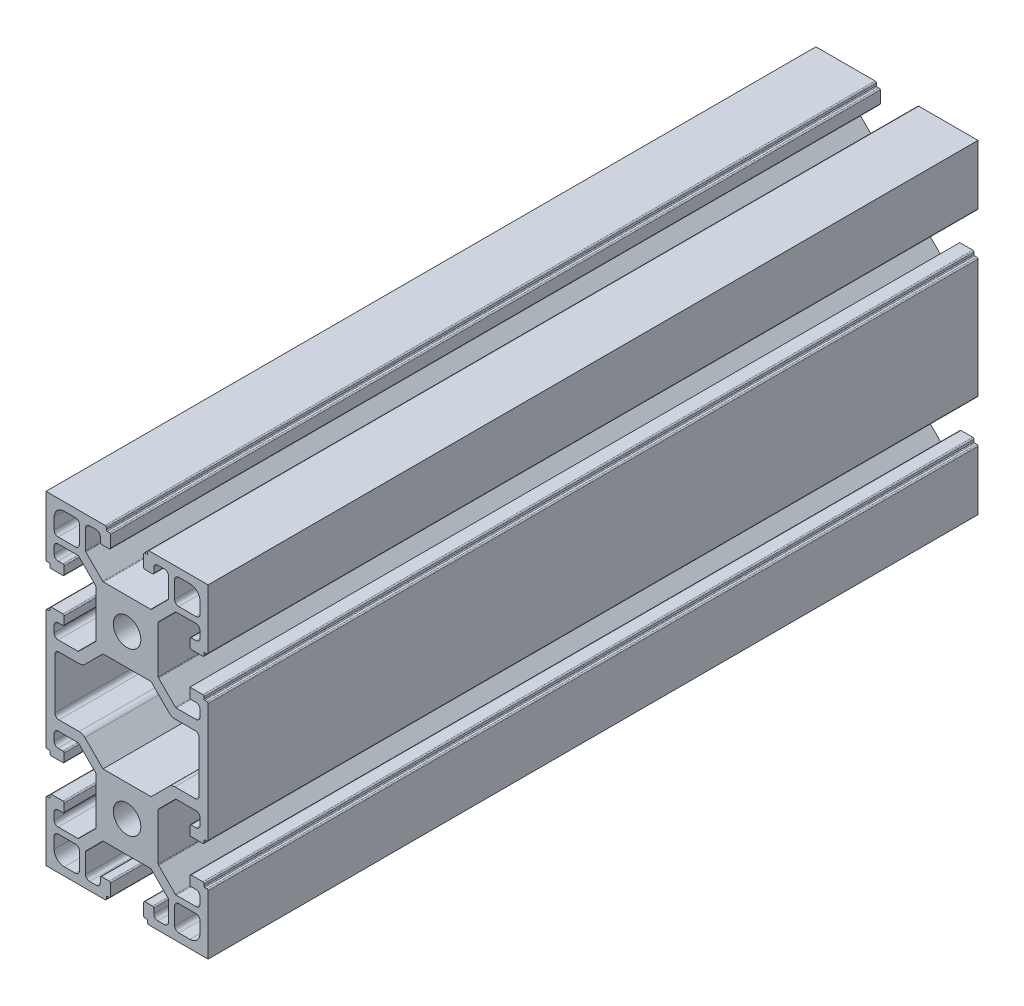
from build123d import *

# Parameters (mm, degrees)
MODEL_R                          = 3.4
EXTRUDE_1_DEPTH                  = 95
HOLE_WIZARD_M8_1_D               = 6.8
HOLE_WIZARD_M8_1_DEPTH           = 19.75
HOLE_WIZARD_M8_1_TIP             = 2.042926105
HOLE_WIZARD_M8_1_ON_FACE_2_D     = 6.8
HOLE_WIZARD_M8_1_ON_FACE_2_DEPTH = 19.75
HOLE_WIZARD_M8_1_ON_FACE_2_TIP   = 2.042926105


with BuildPart() as part:
    # Model → 凸台-拉伸1 (new, symmetric)
    with BuildSketch(Plane.XY):
        with BuildLine():
            Line((714.409918253, 268.229784956), (714.409918253, 266.329784956))
            ThreePointArc((714.409918253, 266.329784956), (714.322050287, 266.117652922), (714.109918253, 266.029784956))
            Line((714.109918253, 266.029784956), (711.209918253, 266.029784956))
            ThreePointArc((711.209918253, 266.029784956), (710.997786218, 266.117652922), (710.909918253, 266.329784956))
            Line((710.909918253, 266.329784956), (710.909918253, 266.829784956))
            ThreePointArc((710.909918253, 266.829784956), (710.851339609, 266.971206313), (710.709918253, 267.029784956))
            Line((710.709918253, 267.029784956), (710.209918253, 267.029784956))
            ThreePointArc((710.209918253, 267.029784956), (709.997786218, 267.117652922), (709.909918253, 267.329784956))
            Line((709.909918253, 267.329784956), (709.909918253, 281.929784956))
            Line((709.909918253, 281.929784956), (724.509918253, 281.929784956))
            ThreePointArc((724.509918253, 281.929784956), (724.722050287, 281.841916991), (724.809918253, 281.629784956))
            Line((724.809918253, 281.629784956), (724.809918253, 281.129784956))
            ThreePointArc((724.809918253, 281.129784956), (724.868496896, 280.9883636), (725.009918253, 280.929784956))
            Line((725.009918253, 280.929784956), (725.509918253, 280.929784956))
            ThreePointArc((725.509918253, 280.929784956), (725.722050287, 280.841916991), (725.809918253, 280.629784956))
            Line((725.809918253, 280.629784956), (725.809918253, 277.729784956))
            ThreePointArc((725.809918253, 277.729784956), (725.722050287, 277.517652922), (725.509918253, 277.429784956))
            Line((725.509918253, 277.429784956), (723.609918253, 277.429784956))
            ThreePointArc((723.609918253, 277.429784956), (723.397786218, 277.517652922), (723.309918253, 277.729784956))
            Line((723.309918253, 277.729784956), (723.309918253, 278.929784956))
            ThreePointArc((723.309918253, 278.929784956), (723.017025034, 279.636891738), (722.309918253, 279.929784956))
            Line((722.309918253, 279.929784956), (720.659918253, 279.929784956))
            ThreePointArc((720.659918253, 279.929784956), (719.952811471, 279.636891738), (719.659918253, 278.929784956))
            Line((719.659918253, 278.929784956), (719.659918253, 274.071815978))
            ThreePointArc((719.659918253, 274.071815978), (719.682754393, 273.957010948), (719.747786218, 273.859683944))
            Line((719.747786218, 273.859683944), (723.88981724, 269.717652922))
            ThreePointArc((723.88981724, 269.717652922), (723.987144245, 269.652621097), (724.101949274, 269.629784956))
            Line((724.101949274, 269.629784956), (735.717887231, 269.629784956))
            ThreePointArc((735.717887231, 269.629784956), (735.832692261, 269.652621097), (735.930019265, 269.717652922))
            Line((735.930019265, 269.717652922), (740.072050287, 273.859683944))
            ThreePointArc((740.072050287, 273.859683944), (740.137082112, 273.957010948), (740.159918253, 274.071815978))
            Line((740.159918253, 274.071815978), (740.159918253, 278.929784956))
            ThreePointArc((740.159918253, 278.929784956), (739.867025034, 279.636891738), (739.159918253, 279.929784956))
            Line((739.159918253, 279.929784956), (737.509918253, 279.929784956))
            ThreePointArc((737.509918253, 279.929784956), (736.802811471, 279.636891738), (736.509918253, 278.929784956))
            Line((736.509918253, 278.929784956), (736.509918253, 277.729784956))
            ThreePointArc((736.509918253, 277.729784956), (736.422050287, 277.517652922), (736.209918253, 277.429784956))
            Line((736.209918253, 277.429784956), (734.309918253, 277.429784956))
            ThreePointArc((734.309918253, 277.429784956), (734.097786218, 277.517652922), (734.009918253, 277.729784956))
            Line((734.009918253, 277.729784956), (734.009918253, 280.629784956))
            ThreePointArc((734.009918253, 280.629784956), (734.097786218, 280.841916991), (734.309918253, 280.929784956))
            Line((734.309918253, 280.929784956), (734.809918253, 280.929784956))
            ThreePointArc((734.809918253, 280.929784956), (734.951339609, 280.9883636), (735.009918253, 281.129784956))
            Line((735.009918253, 281.129784956), (735.009918253, 281.629784956))
            ThreePointArc((735.009918253, 281.629784956), (735.097786218, 281.841916991), (735.309918253, 281.929784956))
            Line((735.309918253, 281.929784956), (749.909918253, 281.929784956))
            Line((749.909918253, 281.929784956), (749.909918253, 267.329784956))
            ThreePointArc((749.909918253, 267.329784956), (749.822050287, 267.117652922), (749.609918253, 267.029784956))
            Line((749.609918253, 267.029784956), (749.109918253, 267.029784956))
            ThreePointArc((749.109918253, 267.029784956), (748.968496896, 266.971206313), (748.909918253, 266.829784956))
            Line((748.909918253, 266.829784956), (748.909918253, 266.329784956))
            ThreePointArc((748.909918253, 266.329784956), (748.822050287, 266.117652922), (748.609918253, 266.029784956))
            Line((748.609918253, 266.029784956), (745.709918253, 266.029784956))
            ThreePointArc((745.709918253, 266.029784956), (745.497786218, 266.117652922), (745.409918253, 266.329784956))
            Line((745.409918253, 266.329784956), (745.409918253, 268.229784956))
            ThreePointArc((745.409918253, 268.229784956), (745.497786218, 268.441916991), (745.709918253, 268.529784956))
            Line((745.709918253, 268.529784956), (746.909918253, 268.529784956))
            ThreePointArc((746.909918253, 268.529784956), (747.617025034, 268.822678175), (747.909918253, 269.529784956))
            Line((747.909918253, 269.529784956), (747.909918253, 271.179784956))
            ThreePointArc((747.909918253, 271.179784956), (747.617025034, 271.886891738), (746.909918253, 272.179784956))
            Line((746.909918253, 272.179784956), (742.051949274, 272.179784956))
            ThreePointArc((742.051949274, 272.179784956), (741.937144245, 272.156948816), (741.83981724, 272.091916991))
            Line((741.83981724, 272.091916991), (737.697786218, 267.949885969))
            ThreePointArc((737.697786218, 267.949885969), (737.632754393, 267.852558964), (737.609918253, 267.737753935))
            Line((737.609918253, 267.737753935), (737.609918253, 256.121815978))
            ThreePointArc((737.609918253, 256.121815978), (737.632754393, 256.007010948), (737.697786218, 255.909683944))
            Line((737.697786218, 255.909683944), (741.83981724, 251.767652922))
            ThreePointArc((741.83981724, 251.767652922), (741.937144245, 251.702621097), (742.051949274, 251.679784956))
            Line((742.051949274, 251.679784956), (746.909918253, 251.679784956))
            ThreePointArc((746.909918253, 251.679784956), (747.617025034, 251.972678175), (747.909918253, 252.679784956))
            Line((747.909918253, 252.679784956), (747.909918253, 254.329784956))
            ThreePointArc((747.909918253, 254.329784956), (747.617025034, 255.036891738), (746.909918253, 255.329784956))
            Line((746.909918253, 255.329784956), (745.409918253, 255.329784956))
            Line((745.409918253, 255.329784956), (745.409918253, 257.829784956))
            Line((745.409918253, 257.829784956), (748.609918253, 257.829784956))
            ThreePointArc((748.609918253, 257.829784956), (748.822050287, 257.741916991), (748.909918253, 257.529784956))
            Line((748.909918253, 257.529784956), (748.909918253, 257.029784956))
            ThreePointArc((748.909918253, 257.029784956), (748.968496896, 256.8883636), (749.109918253, 256.829784956))
            Line((749.109918253, 256.829784956), (749.609918253, 256.829784956))
            ThreePointArc((749.609918253, 256.829784956), (749.822050287, 256.741916991), (749.909918253, 256.529784956))
            Line((749.909918253, 256.529784956), (749.909918253, 241.929784956))
            Line((749.909918253, 241.929784956), (749.909918253, 227.329784956))
            ThreePointArc((749.909918253, 227.329784956), (749.822050287, 227.117652922), (749.609918253, 227.029784956))
            Line((749.609918253, 227.029784956), (749.109918253, 227.029784956))
            ThreePointArc((749.109918253, 227.029784956), (748.968496896, 226.971206313), (748.909918253, 226.829784956))
            Line((748.909918253, 226.829784956), (748.909918253, 226.329784956))
            ThreePointArc((748.909918253, 226.329784956), (748.822050287, 226.117652922), (748.609918253, 226.029784956))
            Line((748.609918253, 226.029784956), (745.709918253, 226.029784956))
            ThreePointArc((745.709918253, 226.029784956), (745.497786218, 226.117652922), (745.409918253, 226.329784956))
            Line((745.409918253, 226.329784956), (745.409918253, 228.229784956))
            ThreePointArc((745.409918253, 228.229784956), (745.497786218, 228.441916991), (745.709918253, 228.529784956))
            Line((745.709918253, 228.529784956), (746.909918253, 228.529784956))
            ThreePointArc((746.909918253, 228.529784956), (747.617025034, 228.822678175), (747.909918253, 229.529784956))
            Line((747.909918253, 229.529784956), (747.909918253, 231.179784956))
            ThreePointArc((747.909918253, 231.179784956), (747.617025034, 231.886891738), (746.909918253, 232.179784956))
            Line((746.909918253, 232.179784956), (742.051949274, 232.179784956))
            ThreePointArc((742.051949274, 232.179784956), (741.937144245, 232.156948816), (741.83981724, 232.091916991))
            Line((741.83981724, 232.091916991), (737.697786218, 227.949885969))
            ThreePointArc((737.697786218, 227.949885969), (737.632754393, 227.852558964), (737.609918253, 227.737753935))
            Line((737.609918253, 227.737753935), (737.609918253, 216.121815978))
            ThreePointArc((737.609918253, 216.121815978), (737.632754393, 216.007010948), (737.697786218, 215.909683944))
            Line((737.697786218, 215.909683944), (741.83981724, 211.767652922))
            ThreePointArc((741.83981724, 211.767652922), (741.937144245, 211.702621097), (742.051949274, 211.679784956))
            Line((742.051949274, 211.679784956), (746.909918253, 211.679784956))
            ThreePointArc((746.909918253, 211.679784956), (747.617025034, 211.972678175), (747.909918253, 212.679784956))
            Line((747.909918253, 212.679784956), (747.909918253, 214.329784956))
            ThreePointArc((747.909918253, 214.329784956), (747.617025034, 215.036891738), (746.909918253, 215.329784956))
            Line((746.909918253, 215.329784956), (745.709918253, 215.329784956))
            ThreePointArc((745.709918253, 215.329784956), (745.497786218, 215.417652922), (745.409918253, 215.629784956))
            Line((745.409918253, 215.629784956), (745.409918253, 217.529784956))
            ThreePointArc((745.409918253, 217.529784956), (745.497786218, 217.741916991), (745.709918253, 217.829784956))
            Line((745.709918253, 217.829784956), (748.609918253, 217.829784956))
            ThreePointArc((748.609918253, 217.829784956), (748.822050287, 217.741916991), (748.909918253, 217.529784956))
            Line((748.909918253, 217.529784956), (748.909918253, 217.029784956))
            ThreePointArc((748.909918253, 217.029784956), (748.968496896, 216.8883636), (749.109918253, 216.829784956))
            Line((749.109918253, 216.829784956), (749.609918253, 216.829784956))
            ThreePointArc((749.609918253, 216.829784956), (749.822050287, 216.741916991), (749.909918253, 216.529784956))
            Line((749.909918253, 216.529784956), (749.909918253, 201.929784956))
            Line((749.909918253, 201.929784956), (735.309918253, 201.929784956))
            ThreePointArc((735.309918253, 201.929784956), (735.097786218, 202.017652922), (735.009918253, 202.229784956))
            Line((735.009918253, 202.229784956), (735.009918253, 202.729784956))
            ThreePointArc((735.009918253, 202.729784956), (734.951339609, 202.871206313), (734.809918253, 202.929784956))
            Line((734.809918253, 202.929784956), (734.309918253, 202.929784956))
            ThreePointArc((734.309918253, 202.929784956), (734.097786218, 203.017652922), (734.009918253, 203.229784956))
            Line((734.009918253, 203.229784956), (734.009918253, 206.129784956))
            ThreePointArc((734.009918253, 206.129784956), (734.097786218, 206.341916991), (734.309918253, 206.429784956))
            Line((734.309918253, 206.429784956), (736.209918253, 206.429784956))
            ThreePointArc((736.209918253, 206.429784956), (736.422050287, 206.341916991), (736.509918253, 206.129784956))
            Line((736.509918253, 206.129784956), (736.509918253, 204.929784956))
            ThreePointArc((736.509918253, 204.929784956), (736.802811471, 204.222678175), (737.509918253, 203.929784956))
            Line((737.509918253, 203.929784956), (739.159918253, 203.929784956))
            ThreePointArc((739.159918253, 203.929784956), (739.867025034, 204.222678175), (740.159918253, 204.929784956))
            Line((740.159918253, 204.929784956), (740.159918253, 209.787753935))
            ThreePointArc((740.159918253, 209.787753935), (740.137082112, 209.902558964), (740.072050287, 209.999885969))
            Line((740.072050287, 209.999885969), (735.930019265, 214.141916991))
            ThreePointArc((735.930019265, 214.141916991), (735.832692261, 214.206948816), (735.717887231, 214.229784956))
            Line((735.717887231, 214.229784956), (724.101949274, 214.229784956))
            ThreePointArc((724.101949274, 214.229784956), (723.987144245, 214.206948816), (723.88981724, 214.141916991))
            Line((723.88981724, 214.141916991), (719.747786218, 209.999885969))
            ThreePointArc((719.747786218, 209.999885969), (719.682754393, 209.902558964), (719.659918253, 209.787753935))
            Line((719.659918253, 209.787753935), (719.659918253, 204.929784956))
            ThreePointArc((719.659918253, 204.929784956), (719.952811471, 204.222678175), (720.659918253, 203.929784956))
            Line((720.659918253, 203.929784956), (722.309918253, 203.929784956))
            ThreePointArc((722.309918253, 203.929784956), (723.017025034, 204.222678175), (723.309918253, 204.929784956))
            Line((723.309918253, 204.929784956), (723.309918253, 206.129784956))
            ThreePointArc((723.309918253, 206.129784956), (723.397786218, 206.341916991), (723.609918253, 206.429784956))
            Line((723.609918253, 206.429784956), (725.509918253, 206.429784956))
            ThreePointArc((725.509918253, 206.429784956), (725.722050287, 206.341916991), (725.809918253, 206.129784956))
            Line((725.809918253, 206.129784956), (725.809918253, 203.229784956))
            ThreePointArc((725.809918253, 203.229784956), (725.722050287, 203.017652922), (725.509918253, 202.929784956))
            Line((725.509918253, 202.929784956), (725.009918253, 202.929784956))
            ThreePointArc((725.009918253, 202.929784956), (724.868496896, 202.871206313), (724.809918253, 202.729784956))
            Line((724.809918253, 202.729784956), (724.809918253, 202.229784956))
            ThreePointArc((724.809918253, 202.229784956), (724.722050287, 202.017652922), (724.509918253, 201.929784956))
            Line((724.509918253, 201.929784956), (709.909918253, 201.929784956))
            Line((709.909918253, 201.929784956), (709.909918253, 216.529784956))
            ThreePointArc((709.909918253, 216.529784956), (709.997786218, 216.741916991), (710.209918253, 216.829784956))
            Line((710.209918253, 216.829784956), (710.709918253, 216.829784956))
            ThreePointArc((710.709918253, 216.829784956), (710.851339609, 216.8883636), (710.909918253, 217.029784956))
            Line((710.909918253, 217.029784956), (710.909918253, 217.529784956))
            ThreePointArc((710.909918253, 217.529784956), (710.997786218, 217.741916991), (711.209918253, 217.829784956))
            Line((711.209918253, 217.829784956), (714.109918253, 217.829784956))
            ThreePointArc((714.109918253, 217.829784956), (714.322050287, 217.741916991), (714.409918253, 217.529784956))
            Line((714.409918253, 217.529784956), (714.409918253, 215.629784956))
            ThreePointArc((714.409918253, 215.629784956), (714.322050287, 215.417652922), (714.109918253, 215.329784956))
            Line((714.109918253, 215.329784956), (712.909918253, 215.329784956))
            ThreePointArc((712.909918253, 215.329784956), (712.202811471, 215.036891738), (711.909918253, 214.329784956))
            Line((711.909918253, 214.329784956), (711.909918253, 212.679784956))
            ThreePointArc((711.909918253, 212.679784956), (712.202811471, 211.972678175), (712.909918253, 211.679784956))
            Line((712.909918253, 211.679784956), (717.767887231, 211.679784956))
            ThreePointArc((717.767887231, 211.679784956), (717.882692261, 211.702621097), (717.980019265, 211.767652922))
            Line((717.980019265, 211.767652922), (722.122050287, 215.909683944))
            ThreePointArc((722.122050287, 215.909683944), (722.187082112, 216.007010948), (722.209918253, 216.121815978))
            Line((722.209918253, 216.121815978), (722.209918253, 227.737753935))
            ThreePointArc((722.209918253, 227.737753935), (722.187082112, 227.852558964), (722.122050287, 227.949885969))
            Line((722.122050287, 227.949885969), (717.980019265, 232.091916991))
            ThreePointArc((717.980019265, 232.091916991), (717.882692261, 232.156948816), (717.767887231, 232.179784956))
            Line((717.767887231, 232.179784956), (712.909918253, 232.179784956))
            ThreePointArc((712.909918253, 232.179784956), (712.202811471, 231.886891738), (711.909918253, 231.179784956))
            Line((711.909918253, 231.179784956), (711.909918253, 229.529784956))
            ThreePointArc((711.909918253, 229.529784956), (712.202811471, 228.822678175), (712.909918253, 228.529784956))
            Line((712.909918253, 228.529784956), (714.109918253, 228.529784956))
            ThreePointArc((714.109918253, 228.529784956), (714.322050287, 228.441916991), (714.409918253, 228.229784956))
            Line((714.409918253, 228.229784956), (714.409918253, 226.329784956))
            ThreePointArc((714.409918253, 226.329784956), (714.322050287, 226.117652922), (714.109918253, 226.029784956))
            Line((714.109918253, 226.029784956), (711.209918253, 226.029784956))
            ThreePointArc((711.209918253, 226.029784956), (710.997786218, 226.117652922), (710.909918253, 226.329784956))
            Line((710.909918253, 226.329784956), (710.909918253, 226.829784956))
            ThreePointArc((710.909918253, 226.829784956), (710.851339609, 226.971206313), (710.709918253, 227.029784956))
            Line((710.709918253, 227.029784956), (710.209918253, 227.029784956))
            ThreePointArc((710.209918253, 227.029784956), (709.997786218, 227.117652922), (709.909918253, 227.329784956))
            Line((709.909918253, 227.329784956), (709.909918253, 241.929784956))
            Line((709.909918253, 241.929784956), (709.909918253, 256.529784956))
            ThreePointArc((709.909918253, 256.529784956), (709.997786218, 256.741916991), (710.209918253, 256.829784956))
            Line((710.209918253, 256.829784956), (710.709918253, 256.829784956))
            ThreePointArc((710.709918253, 256.829784956), (710.851339609, 256.8883636), (710.909918253, 257.029784956))
            Line((710.909918253, 257.029784956), (710.909918253, 257.529784956))
            ThreePointArc((710.909918253, 257.529784956), (710.997786218, 257.741916991), (711.209918253, 257.829784956))
            Line((711.209918253, 257.829784956), (714.109918253, 257.829784956))
            ThreePointArc((714.109918253, 257.829784956), (714.322050287, 257.741916991), (714.409918253, 257.529784956))
            Line((714.409918253, 257.529784956), (714.409918253, 255.629784956))
            ThreePointArc((714.409918253, 255.629784956), (714.322050287, 255.417652922), (714.109918253, 255.329784956))
            Line((714.109918253, 255.329784956), (712.909918253, 255.329784956))
            ThreePointArc((712.909918253, 255.329784956), (712.202811471, 255.036891738), (711.909918253, 254.329784956))
            Line((711.909918253, 254.329784956), (711.909918253, 252.679784956))
            ThreePointArc((711.909918253, 252.679784956), (712.202811471, 251.972678175), (712.909918253, 251.679784956))
            Line((712.909918253, 251.679784956), (717.767887231, 251.679784956))
            ThreePointArc((717.767887231, 251.679784956), (717.882692261, 251.702621097), (717.980019265, 251.767652922))
            Line((717.980019265, 251.767652922), (722.122050287, 255.909683944))
            ThreePointArc((722.122050287, 255.909683944), (722.187082112, 256.007010948), (722.209918253, 256.121815978))
            Line((722.209918253, 256.121815978), (722.209918253, 267.737753935))
            ThreePointArc((722.209918253, 267.737753935), (722.187082112, 267.852558964), (722.122050287, 267.949885969))
            Line((722.122050287, 267.949885969), (717.980019265, 272.091916991))
            ThreePointArc((717.980019265, 272.091916991), (717.882692261, 272.156948816), (717.767887231, 272.179784956))
            Line((717.767887231, 272.179784956), (712.909918253, 272.179784956))
            ThreePointArc((712.909918253, 272.179784956), (712.202811471, 271.886891738), (711.909918253, 271.179784956))
            Line((711.909918253, 271.179784956), (711.909918253, 269.529784956))
            ThreePointArc((711.909918253, 269.529784956), (712.202811471, 268.822678175), (712.909918253, 268.529784956))
            Line((712.909918253, 268.529784956), (714.109918253, 268.529784956))
            ThreePointArc((714.109918253, 268.529784956), (714.322050287, 268.441916991), (714.409918253, 268.229784956))
        make_face()
        with Locations((729.909918253, 261.929784956)):
            Circle(MODEL_R, mode=Mode.SUBTRACT)
        with Locations((729.909918253, 221.929784956)):
            Circle(MODEL_R, mode=Mode.SUBTRACT)
        with BuildLine():
            Line((718.099258081, 234.679784956), (713.109918253, 234.679784956))
            ThreePointArc((713.109918253, 234.679784956), (712.402811471, 234.972678175), (712.109918253, 235.679784956))
            Line((712.109918253, 235.679784956), (712.109918253, 241.929784956))
            Line((712.109918253, 241.929784956), (712.109918253, 248.179784956))
            ThreePointArc((712.109918253, 248.179784956), (712.402811471, 248.886891738), (713.109918253, 249.179784956))
            Line((713.109918253, 249.179784956), (718.099258081, 249.179784956))
            ThreePointArc((718.099258081, 249.179784956), (718.864624946, 249.332025891), (719.513471643, 249.765571394))
            Line((719.513471643, 249.765571394), (723.977685206, 254.229784956))
            Line((723.977685206, 254.229784956), (735.8421513, 254.229784956))
            Line((735.8421513, 254.229784956), (740.306364862, 249.765571394))
            ThreePointArc((740.306364862, 249.765571394), (740.95521156, 249.332025891), (741.720578424, 249.179784956))
            Line((741.720578424, 249.179784956), (746.709918253, 249.179784956))
            ThreePointArc((746.709918253, 249.179784956), (747.417025034, 248.886891738), (747.709918253, 248.179784956))
            Line((747.709918253, 248.179784956), (747.709918253, 241.929784956))
            Line((747.709918253, 241.929784956), (747.709918253, 235.679784956))
            ThreePointArc((747.709918253, 235.679784956), (747.417025034, 234.972678175), (746.709918253, 234.679784956))
            Line((746.709918253, 234.679784956), (741.720578424, 234.679784956))
            ThreePointArc((741.720578424, 234.679784956), (740.95521156, 234.527544021), (740.306364862, 234.093998519))
            Line((740.306364862, 234.093998519), (735.8421513, 229.629784956))
            Line((735.8421513, 229.629784956), (723.977685206, 229.629784956))
            Line((723.977685206, 229.629784956), (719.513471643, 234.093998519))
            ThreePointArc((719.513471643, 234.093998519), (718.864624946, 234.527544021), (718.099258081, 234.679784956))
        make_face(mode=Mode.SUBTRACT)
        with BuildLine():
            Line((718.159918253, 278.929784956), (718.159918253, 274.679784956))
            ThreePointArc((718.159918253, 274.679784956), (717.867025034, 273.972678175), (717.159918253, 273.679784956))
            Line((717.159918253, 273.679784956), (712.909918253, 273.679784956))
            ThreePointArc((712.909918253, 273.679784956), (712.202811471, 273.972678175), (711.909918253, 274.679784956))
            Line((711.909918253, 274.679784956), (711.909918253, 277.429784956))
            ThreePointArc((711.909918253, 277.429784956), (712.6421513, 279.197551909), (714.409918252, 279.929784956))
            Line((714.409918252, 279.929784956), (717.159918253, 279.929784956))
            ThreePointArc((717.159918253, 279.929784956), (717.867025034, 279.636891738), (718.159918253, 278.929784956))
        make_face(mode=Mode.SUBTRACT)
        with BuildLine():
            Line((741.659918253, 278.929784956), (741.659918253, 274.679784956))
            ThreePointArc((741.659918253, 274.679784956), (741.952811471, 273.972678175), (742.659918253, 273.679784956))
            Line((742.659918253, 273.679784956), (746.909918253, 273.679784956))
            ThreePointArc((746.909918253, 273.679784956), (747.617025034, 273.972678175), (747.909918253, 274.679784956))
            Line((747.909918253, 274.679784956), (747.909918253, 277.429784956))
            ThreePointArc((747.909918253, 277.429784956), (747.177685206, 279.197551909), (745.409918253, 279.929784956))
            Line((745.409918253, 279.929784956), (742.659918253, 279.929784956))
            ThreePointArc((742.659918253, 279.929784956), (741.952811471, 279.636891738), (741.659918253, 278.929784956))
        make_face(mode=Mode.SUBTRACT)
        with BuildLine():
            Line((711.909918253, 206.429784956), (711.909918253, 209.179784956))
            ThreePointArc((711.909918253, 209.179784956), (712.202811471, 209.886891738), (712.909918253, 210.179784956))
            Line((712.909918253, 210.179784956), (717.159918253, 210.179784956))
            ThreePointArc((717.159918253, 210.179784956), (717.867025034, 209.886891738), (718.159918253, 209.179784956))
            Line((718.159918253, 209.179784956), (718.159918253, 204.929784956))
            ThreePointArc((718.159918253, 204.929784956), (717.867025034, 204.222678175), (717.159918253, 203.929784956))
            Line((717.159918253, 203.929784956), (714.409918252, 203.929784956))
            ThreePointArc((714.409918252, 203.929784956), (712.6421513, 204.662018003), (711.909918253, 206.429784956))
        make_face(mode=Mode.SUBTRACT)
        with BuildLine():
            Line((742.659918253, 203.929784956), (745.409918253, 203.929784956))
            ThreePointArc((745.409918253, 203.929784956), (747.177685206, 204.662018003), (747.909918253, 206.429784956))
            Line((747.909918253, 206.429784956), (747.909918253, 209.179784956))
            ThreePointArc((747.909918253, 209.179784956), (747.617025034, 209.886891738), (746.909918253, 210.179784956))
            Line((746.909918253, 210.179784956), (742.659918253, 210.179784956))
            ThreePointArc((742.659918253, 210.179784956), (741.952811471, 209.886891738), (741.659918253, 209.179784956))
            Line((741.659918253, 209.179784956), (741.659918253, 204.929784956))
            ThreePointArc((741.659918253, 204.929784956), (741.952811471, 204.222678175), (742.659918253, 203.929784956))
        make_face(mode=Mode.SUBTRACT)
    extrude(amount=EXTRUDE_1_DEPTH, both=True)

    # M8 螺纹孔1
    with Locations(Plane(origin=(729.909918253, 261.929784956, 95), x_dir=(1, 0, 0), z_dir=(0, 0, 1))):
        with Locations((0, 0), (0, -40)):
            Hole(HOLE_WIZARD_M8_1_D / 2, depth=HOLE_WIZARD_M8_1_DEPTH)
            with Locations((0, 0, -(HOLE_WIZARD_M8_1_DEPTH + HOLE_WIZARD_M8_1_TIP / 2))):  # 118° drill point
                Cone(0, HOLE_WIZARD_M8_1_D / 2, HOLE_WIZARD_M8_1_TIP, mode=Mode.SUBTRACT)

    # M8 螺纹孔1 on face 2
    with Locations(Plane(origin=(729.909918253, 221.929784956, -95), x_dir=(1, 0, 0), z_dir=(0, 0, 1))):
        with Locations((0, 0), (0, 40)):
            Hole(HOLE_WIZARD_M8_1_ON_FACE_2_D / 2, depth=HOLE_WIZARD_M8_1_ON_FACE_2_DEPTH)
            with Locations((0, 0, -(HOLE_WIZARD_M8_1_ON_FACE_2_DEPTH + HOLE_WIZARD_M8_1_ON_FACE_2_TIP / 2))):  # 118° drill point
                Cone(0, HOLE_WIZARD_M8_1_ON_FACE_2_D / 2, HOLE_WIZARD_M8_1_ON_FACE_2_TIP, mode=Mode.SUBTRACT)


solid = part.part
